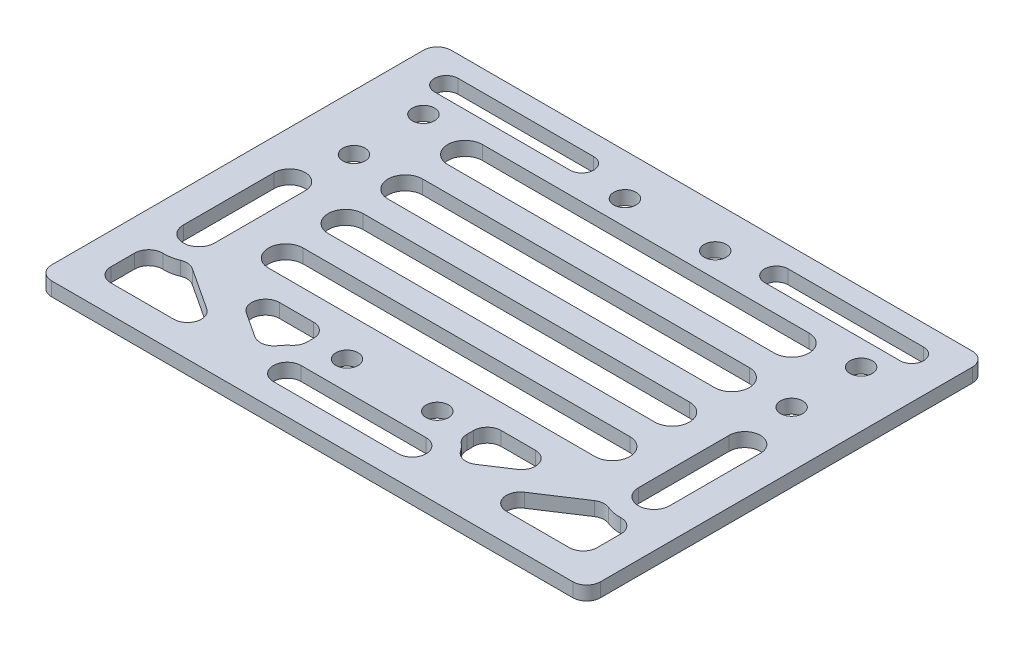
from build123d import *

# Parameters (mm, degrees)
SKETCH1_W           = 79
SKETCH1_H           = 57.5
SKETCH1_R           = 1.6
BOSS_EXTRUDE1_DEPTH = 2
CUT_EXTRUDE1_DEPTH  = 49.895935414
R2_FILLET_1_R       = 2


with BuildPart() as part:
    # Sketch1 → Boss-Extrude1 (new body)
    with BuildSketch(Plane(origin=(0, 0, 0), x_dir=(1, 0, 0), z_dir=(0, 1, 0))):
        Rectangle(SKETCH1_W, SKETCH1_H)
        with Locations(Location((-31.5, 18.75, 0), (0, 0, 270))):
            Circle(SKETCH1_R, mode=Mode.SUBTRACT)
        with Locations(Location((-31.5, 8.75, 0), (0, 0, 270))):
            Circle(SKETCH1_R, mode=Mode.SUBTRACT)
        with Locations(Location((31.5, 8.75, 0), (0, 0, 90))):
            Circle(SKETCH1_R, mode=Mode.SUBTRACT)
        with Locations(Location((31.5, 18.75, 0), (0, 0, 90))):
            Circle(SKETCH1_R, mode=Mode.SUBTRACT)
        with Locations(Location((-6.5, 22.75, 0), (0, 0, 270))):
            Circle(SKETCH1_R, mode=Mode.SUBTRACT)
        with Locations(Location((-6.5, -17.25, 0), (0, 0, 270))):
            Circle(SKETCH1_R, mode=Mode.SUBTRACT)
        with Locations(Location((6.5, 22.75, 0), (0, 0, 90))):
            Circle(SKETCH1_R, mode=Mode.SUBTRACT)
        with Locations(Location((6.5, -17.25, 0), (0, 0, 90))):
            Circle(SKETCH1_R, mode=Mode.SUBTRACT)
    extrude(amount=BOSS_EXTRUDE1_DEPTH)

    # Sketch2 → Cut-Extrude1 (cut, through all)
    with BuildSketch(Plane(origin=(0, 2, 0), x_dir=(1, 0, 0), z_dir=(0, 1, 0))):
        with BuildLine():
            Line((-23.5, 19.25), (23.5, 19.25))
            ThreePointArc((23.5, 19.25), (26, 16.75), (23.5, 14.25))
            Line((23.5, 14.25), (-23.5, 14.25))
            ThreePointArc((-23.5, 14.25), (-26, 16.75), (-23.5, 19.25))
        make_face()
        with BuildLine():
            Line((-23.5, 10.65), (23.5, 10.65))
            ThreePointArc((23.5, 10.65), (26, 8.15), (23.5, 5.65))
            Line((23.5, 5.65), (-23.5, 5.65))
            ThreePointArc((-23.5, 5.65), (-26, 8.15), (-23.5, 10.65))
        make_face()
        with BuildLine():
            Line((-23.5, 2.05), (23.5, 2.05))
            ThreePointArc((23.5, 2.05), (26, -0.45), (23.5, -2.95))
            Line((23.5, -2.95), (-23.5, -2.95))
            ThreePointArc((-23.5, -2.95), (-26, -0.45), (-23.5, 2.05))
        make_face()
        with BuildLine():
            Line((-23.5, -6.55), (23.5, -6.55))
            ThreePointArc((23.5, -6.55), (26, -9.05), (23.5, -11.55))
            Line((23.5, -11.55), (-23.5, -11.55))
            ThreePointArc((-23.5, -11.55), (-26, -9.05), (-23.5, -6.55))
        make_face()
        with BuildLine():
            Line((-33.5, 25.75), (-14, 25.75))
            ThreePointArc((-14, 25.75), (-12.3, 24.05), (-14, 22.35))
            Line((-14, 22.35), (-33.5, 22.35))
            ThreePointArc((-33.5, 22.35), (-35.2, 24.05), (-33.5, 25.75))
        make_face()
        with BuildLine():
            Line((33.5, 25.75), (14, 25.75))
            ThreePointArc((14, 25.75), (12.3, 24.05), (14, 22.35))
            Line((14, 22.35), (33.5, 22.35))
            ThreePointArc((33.5, 22.35), (35.2, 24.05), (33.5, 25.75))
        make_face()
        with BuildLine():
            Line((-9, -21.35), (9, -21.35))
            ThreePointArc((9, -21.35), (11, -23.35), (9, -25.35))
            Line((9, -25.35), (-9, -25.35))
            ThreePointArc((-9, -25.35), (-11, -23.35), (-9, -21.35))
        make_face()
        with BuildLine():
            Line((-30.5, 0.75), (-30.5, -12.305379368))
            ThreePointArc((-30.5, -12.305379368), (-32.75, -14.555379368), (-35, -12.305379368))
            Line((-35, -12.305379368), (-35, 0.75))
            ThreePointArc((-35, 0.75), (-32.75, 3), (-30.5, 0.75))
        make_face()
        with BuildLine():
            Line((30.5, 0.75), (30.5, -12.305379368))
            ThreePointArc((30.5, -12.305379368), (32.75, -14.555379368), (35, -12.305379368))
            Line((35, -12.305379368), (35, 0.75))
            ThreePointArc((35, 0.75), (32.75, 3), (30.5, 0.75))
        make_face()
        with BuildLine():
            Line((-35, -16.770522143), (-35, -24.75))
            Line((-35, -24.75), (-17.261316253, -24.75))
            Line((-17.261316253, -24.75), (-29.927103479, -16.432273507))
            ThreePointArc((-29.927103479, -16.432273507), (-32.417350574, -17.294301533), (-35, -16.770522143))
        make_face()
        with BuildLine():
            Line((-25.10932284, -15.05), (-11.5, -15.05))
            Line((-11.5, -15.05), (-11.5, -19.019872981))
            ThreePointArc((-11.5, -19.019872981), (-13.073188505, -20.450149072), (-13.909844854, -22.404789172))
            Line((-13.909844854, -22.404789172), (-25.10932284, -15.05))
        make_face()
        with BuildLine():
            Line((17.261316253, -24.75), (29.927103479, -16.432273507))
            ThreePointArc((29.927103479, -16.432273507), (32.417350574, -17.294301533), (35, -16.770522143))
            Line((35, -16.770522143), (35, -24.75))
            Line((35, -24.75), (17.261316253, -24.75))
        make_face()
        with BuildLine():
            Line((25.10932284, -15.05), (11.5, -15.05))
            Line((11.5, -15.05), (11.5, -19.019872981))
            ThreePointArc((11.5, -19.019872981), (13.073188505, -20.450149072), (13.909844854, -22.404789172))
            Line((13.909844854, -22.404789172), (25.10932284, -15.05))
        make_face()
    extrude(amount=-CUT_EXTRUDE1_DEPTH, mode=Mode.SUBTRACT)

    # R2 Fillet 1
    r2_fillet_1_edges = [part.edges().sort_by_distance(p)[0] for p in [
        (-11.5, 1, 15.05),
        (-11.5, 1, 19.019872981),
        (-13.909844854, 1, 22.404789172),
        (-25.10932284, 1, 15.05),
        (-35, 1, 16.770522143),
        (-29.927103479, 1, 16.432273507),
        (-17.261316253, 1, 24.75),
        (-35, 1, 24.75),
        (25.10932284, 1, 15.05),
        (13.909844854, 1, 22.404789172),
        (11.5, 1, 19.019872981),
        (11.5, 1, 15.05),
        (29.927103479, 1, 16.432273507),
        (35, 1, 16.770522143),
        (35, 1, 24.75),
        (17.261316253, 1, 24.75),
        (39.5, 1, 28.75),
        (-39.5, 1, 28.75),
        (-39.5, 1, -28.75),
        (39.5, 1, -28.75),
    ]]
    fillet(r2_fillet_1_edges, radius=R2_FILLET_1_R)


solid = part.part
